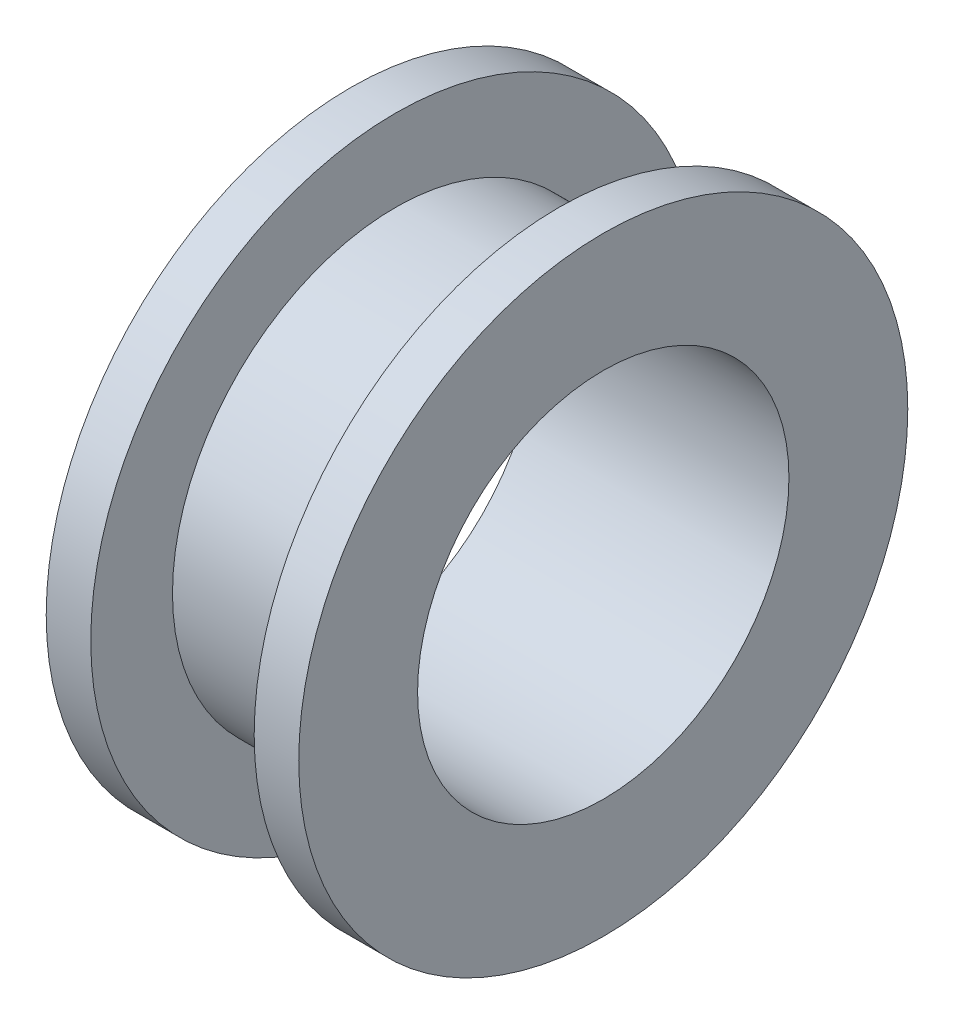
SolidWorks part; units mm, degrees
ref_plane "前视基准面" through (0, 0, 0) normal (0, 0, 1) x (1, 0, 0)
ref_plane "上视基准面" through (0, 0, 0) normal (0, 1, 0) x (1, 0, 0)
ref_plane "右视基准面" through (0, 0, 0) normal (1, 0, 0) x (0, 0, -1)
sketch "草图1" plane through (0, 0, 0) normal (0, 0, 1) x (1, 0, 0)
  line L0 (0, 25) -> (0, 41)
  line L1 (0, 41) -> (6, 41)
  line L2 (6, 41) -> (6, 30)
  line L3 (6, 30) -> (28, 30)
  line L4 (28, 30) -> (28, 41)
  line L5 (28, 41) -> (34, 41)
  line L6 (34, 41) -> (34, 25)
  line L7 (34, 25) -> (0, 25)
  line L8 (0, 0) -> (25.0564, 0) construction
  dimension "D1" = 22
  dimension "D2" = 6
  dimension "D3" = 11
  dimension "D4" = 25
  dimension "D5" = 5
revolve "旋转1" add sketch "草图1" angle 360 about L8
